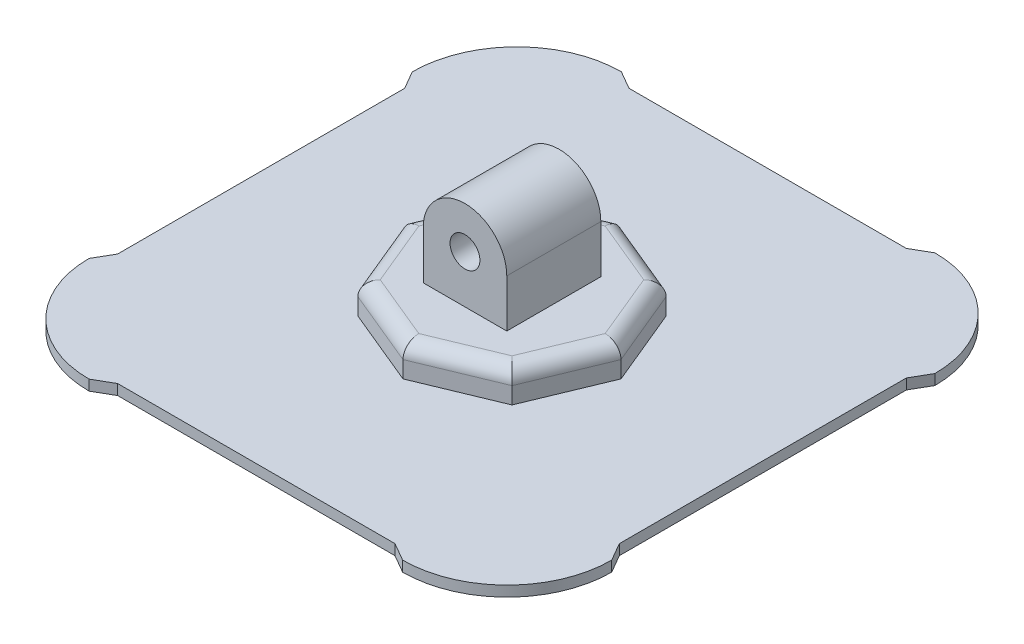
SolidWorks part; units mm, degrees
ref_plane "Front Plane" through (0, 0, 0) normal (0, 0, 1) x (1, 0, 0)
ref_plane "Top Plane" through (0, 0, 0) normal (0, 1, 0) x (1, 0, 0)
ref_plane "Right Plane" through (0, 0, 0) normal (1, 0, 0) x (0, 0, -1)
sketch "Sketch1" plane through (0, 0, 0) normal (0, 1, 0) x (1, 0, 0)
  line L0 (-15, -24.4622) -> (15, -24.4622)
  line L3 (-15, -25.4622) -> (15, -25.4622)
  line L4 (-25, -15.4622) -> (-25, 15.4622)
  line L5 (-15, 25.4622) -> (15, 25.4622)
  line L6 (25, -15.4622) -> (25, 15.4622)
  line L7 (-25, -25.4622) -> (25, 25.4622) construction
  line L8 (-25, 25.4622) -> (25, -25.4622) construction
  line L9 (24, -15.4622) -> (24, 15.4622)
  line L10 (-15, 24.4622) -> (15, 24.4622)
  line L11 (-24, -15.4622) -> (-24, 15.4622)
  line L12 (-25, 15.4622) -> (-24, 13.7301)
  line L13 (-25, 14.78) -> (-22.9249, 14.78) construction
  line L14 (0, 0) -> (-4.3873, 0) construction
  line L15 (-25, -15.4622) -> (-24, -13.7301)
  line L16 (0, 0) -> (0, -4.8391) construction
  line L17 (25, 15.4622) -> (24, 13.7301)
  line L18 (25, -15.4622) -> (24, -13.7301)
  line L19 (-15, -25.4622) -> (-13.2679, -24.4622)
  line L20 (15, -25.4622) -> (13.2679, -24.4622)
  line L21 (-15, 25.4622) -> (-13.2679, 24.4622)
  line L22 (15, 25.4622) -> (13.2679, 24.4622)
  arc A0 (15, -25.4622) -> (25, -15.4622) centre (15, -15.4622) ccw
  arc A1 (-25, 15.4622) -> (-15, 25.4622) centre (-15, 15.4622) cw
  arc A2 (-15, -25.4622) -> (-25, -15.4622) centre (-15, -15.4622) cw
  arc A3 (15, 25.4622) -> (25, 15.4622) centre (15, 15.4622) cw
  arc A4 (15, -24.4622) -> (24, -15.4622) centre (15, -15.4622) ccw construction
  arc A5 (15, 24.4622) -> (24, 15.4622) centre (15, 15.4622) cw construction
  arc A6 (-24, 15.4622) -> (-15, 24.4622) centre (-15, 15.4622) cw construction
  arc A7 (-15, -24.4622) -> (-24, -15.4622) centre (-15, -15.4622) cw construction
  point P0 (0, 0)
  dimension "D3" = 10
  dimension "D1" = 50
  dimension "D2" = 50.9244
  dimension "D4" = 1
  dimension "D5" = 120
  dimension "D6" = 30
extrude "Boss-Extrude1" add sketch "Sketch1" along normal blind 1
sketch "Sketch2" plane through (0, 1, 0) normal (0, 1, 0) x (1, 0, 0)
  line L0 (-10.429, 0) -> (10.429, 0)
  line L1 (-10.429, 0) -> (-7.3744, -7.3744)
  line L2 (-7.3744, -7.3744) -> (0, -10.429)
  line L3 (0, -10.429) -> (7.3744, -7.3744)
  line L4 (7.3744, -7.3744) -> (10.429, 0)
  line L5 (10.429, 0) -> (7.3744, 7.3744)
  line L6 (7.3744, 7.3744) -> (0, 10.429)
  line L7 (0, 10.429) -> (-7.3744, 7.3744)
  line L8 (-7.3744, 7.3744) -> (-10.429, 0)
  circle A0 centre (0, 0) radius 9.6352 construction
extrude "Boss-Extrude2" add sketch "Sketch2" along normal blind 3 contours L3 L4 L0 L1 L2 | L7 L8 L0 L5 L6
fillet "Fillet1" radius 1.4 8 edges at (-3.6872, 4, 8.9017) (-8.9017, 4, 3.6872) (-8.9017, 4, -3.6872) (-3.6872, 4, -8.9017) (3.6872, 4, -8.9017) (8.9017, 4, -3.6872) (8.9017, 4, 3.6872) (3.6872, 4, 8.9017)
sketch "Sketch3" plane through (0, 0, 0) normal (0, 0, 1) x (1, 0, 0)
  line L0 (-3.9859, 8.9043) -> (-3.9859, 4)
  line L1 (0, 8.5691) -> (0, 0) construction
  line L2 (-6.3029, 4) -> (0, 4) construction
  line L3 (4, 8.5691) -> (4, 4)
  line L4 (0, 4) -> (6.3029, 4) construction
  line L5 (-3.9859, 4) -> (4, 4)
  circle A0 centre (0, 8.5691) radius 4
  circle A1 centre (0, 8.5691) radius 1.4263
  dimension "D1" = 8
extrude "Boss-Extrude3" add sketch "Sketch3" along normal mid plane 9
